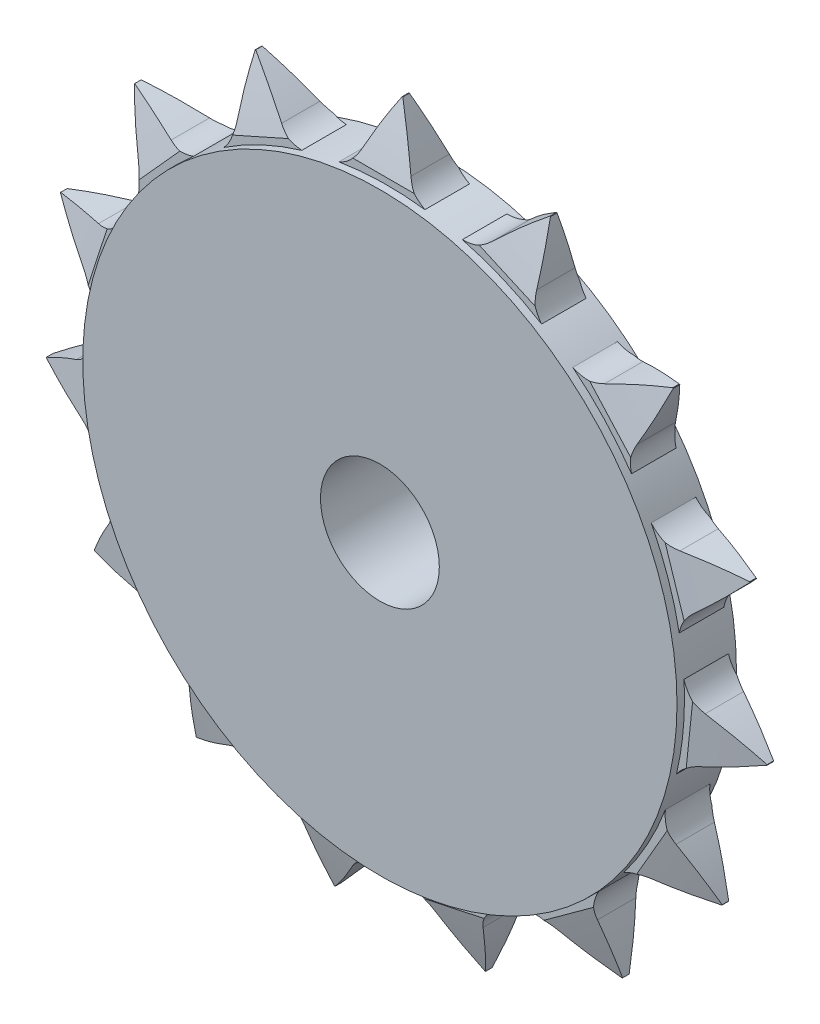
from build123d import *

# Parameters (mm, degrees)
SKETCH1_R           = 5
BOSS_EXTRUDE1_DEPTH = 1
SKETCH2_R           = 3.811759064
BOSS_EXTRUDE2_DEPTH = 0.75
BOSS_EXTRUDE3_DEPTH = 0.375
CUT_EXTRUDE1_DEPTH  = 8.948355434
CIRPATTERN1_COUNT   = 15
SKETCH8_R           = 1
CUT_EXTRUDE2_DEPTH  = 20.75


with BuildPart() as part:
    # Sketch1 → Boss-Extrude1 (new body)
    with BuildSketch(Plane.XY):
        Circle(SKETCH1_R)
    extrude(amount=BOSS_EXTRUDE1_DEPTH)

    # Sketch2 → Boss-Extrude2 (add)
    with BuildSketch(Plane(origin=(0, 0, 0), x_dir=(-1, 0, 0), z_dir=(0, 0, -1))):
        Circle(SKETCH2_R)
    extrude(amount=BOSS_EXTRUDE2_DEPTH)

    # Sketch5 → Boss-Extrude3 (add, symmetric)
    with BuildSketch(Plane.XY.offset(0.5)):
        with BuildLine():
            Line((-0.069046416, 6.097241516), (-0.059046416, 6.097241516))
            ThreePointArc((-0.059046416, 6.097241516), (0.153767594, 5.691926308), (0.345423798, 5.276188265))
            ThreePointArc((0.345423798, 5.276188265), (0.549780197, 5.012820961), (0.859286749, 4.889008325))
            ThreePointArc((0.859286749, 4.889008325), (-0.064046416, 4.941825871), (-0.987305685, 4.887731979))
            ThreePointArc((-0.987305685, 4.887731979), (-0.677595275, 5.012103556), (-0.47351663, 5.276188265))
            ThreePointArc((-0.47351663, 5.276188265), (-0.284693328, 5.693321862), (-0.069046416, 6.097241516))
        make_face()
    boss_extrude3 = extrude(amount=BOSS_EXTRUDE3_DEPTH, both=True)

    # Sketch7 → Cut-Extrude1 (cut, symmetric)
    with BuildSketch(Plane(origin=(0, 0, 0), x_dir=(0, 0, -1), z_dir=(1, 0, 0))):
        with BuildLine():
            Line((-0.55, 6.111195309), (-0.45, 6.111195309))
            ThreePointArc((-0.45, 6.111195309), (-0.282176758, 5.60966822), (-0.125, 5.104703341))
            Line((-0.125, 5.104703341), (0.244003167, 5.104703341))
            Line((0.244003167, 5.104703341), (0.244003167, 6.460555356))
            Line((0.244003167, 6.460555356), (-1.166851933, 6.460555356))
            Line((-1.166851933, 6.460555356), (-1.166851933, 5.104703341))
            Line((-1.166851933, 5.104703341), (-0.875, 5.104703341))
            ThreePointArc((-0.875, 5.104703341), (-0.717823242, 5.60966822), (-0.55, 6.111195309))
        make_face()
    cut_extrude1 = extrude(amount=CUT_EXTRUDE1_DEPTH, both=True, mode=Mode.SUBTRACT)

    # CirPattern1: Boss-Extrude3, Cut-Extrude1 ×15 about axis
    cirpattern1_axis = Axis((0, 0, 0), (0, 0, 1))
    add([boss_extrude3.rotate(cirpattern1_axis, i * 360 / CIRPATTERN1_COUNT) for i in range(1, CIRPATTERN1_COUNT)])
    add([cut_extrude1.rotate(cirpattern1_axis, i * 360 / CIRPATTERN1_COUNT) for i in range(1, CIRPATTERN1_COUNT)], mode=Mode.SUBTRACT)

    # Sketch8 → Cut-Extrude2 (cut)
    with BuildSketch(Plane(origin=(0, 0, -0.75), x_dir=(-1, 0, 0), z_dir=(0, 0, -1))):
        Circle(SKETCH8_R)
    extrude(amount=-CUT_EXTRUDE2_DEPTH, mode=Mode.SUBTRACT)


solid = part.part
